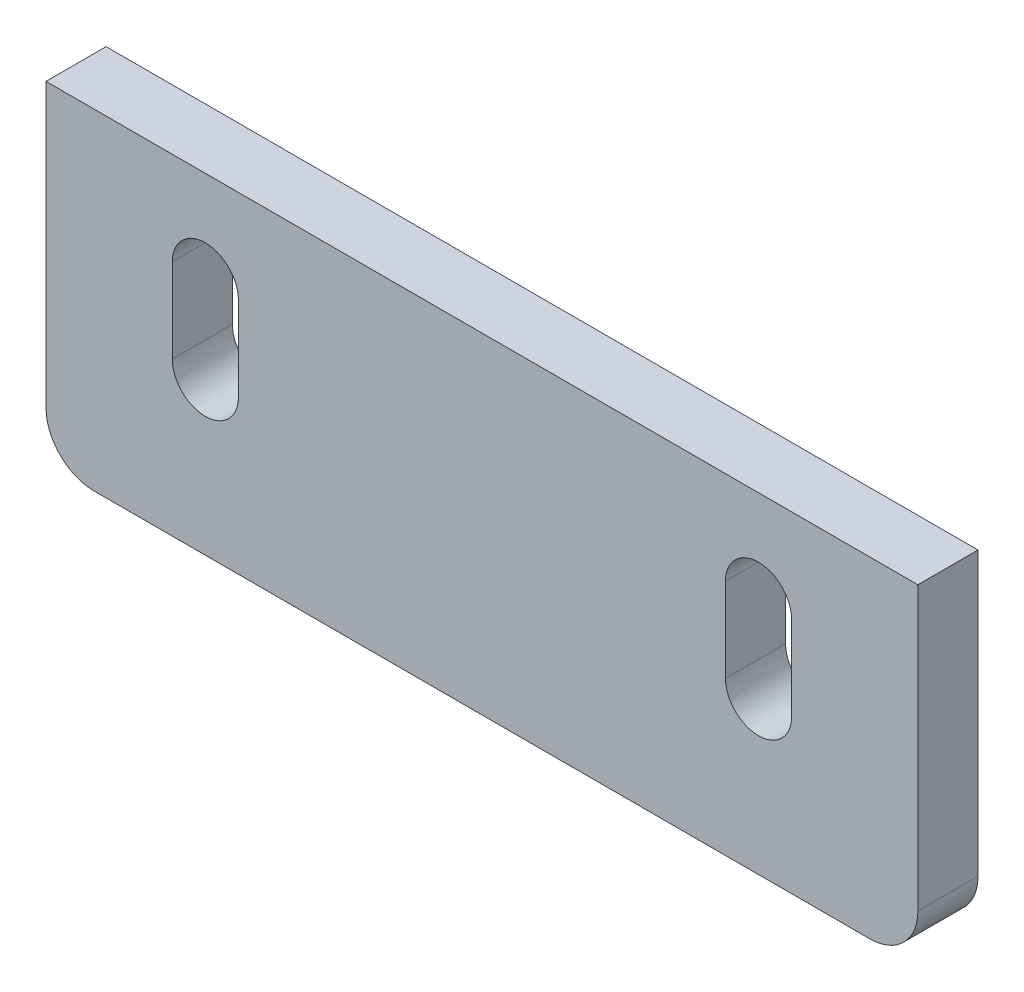
from build123d import *

# Parameters (mm, degrees)
SKETCH_1_W          = 145
SKETCH_1_H          = 55
EXTRUDE_1_DEPTH     = 10
FILLET_1_R          = 8
CUT_EXTRUDE_1_DEPTH = 10


with BuildPart() as part:
    # 草图1 → 凸台-拉伸1 (new body)
    with BuildSketch(Plane.XY):
        Rectangle(SKETCH_1_W, SKETCH_1_H)
    extrude(amount=EXTRUDE_1_DEPTH)

    # 圆角1
    fillet_1_edges = [part.edges().sort_by_distance(p)[0] for p in [
        (72.5, -27.5, 5),
        (-72.5, -27.5, 5),
    ]]
    fillet(fillet_1_edges, radius=FILLET_1_R)

    # 草图2 → 切除-拉伸1 (cut)
    with BuildSketch(Plane.XY.offset(10)):
        with BuildLine():
            Line((51.5, 12), (51.5, -2))
            ThreePointArc((51.5, -2), (46, -7.5), (40.5, -2))
            Line((40.5, -2), (40.5, 12))
            ThreePointArc((40.5, 12), (46, 17.5), (51.5, 12))
        make_face()
        with BuildLine():
            Line((-40.5, 12), (-40.5, -2))
            ThreePointArc((-40.5, -2), (-46, -7.5), (-51.5, -2))
            Line((-51.5, -2), (-51.5, 12))
            ThreePointArc((-51.5, 12), (-46, 17.5), (-40.5, 12))
        make_face()
    extrude(amount=-CUT_EXTRUDE_1_DEPTH, mode=Mode.SUBTRACT)


solid = part.part
